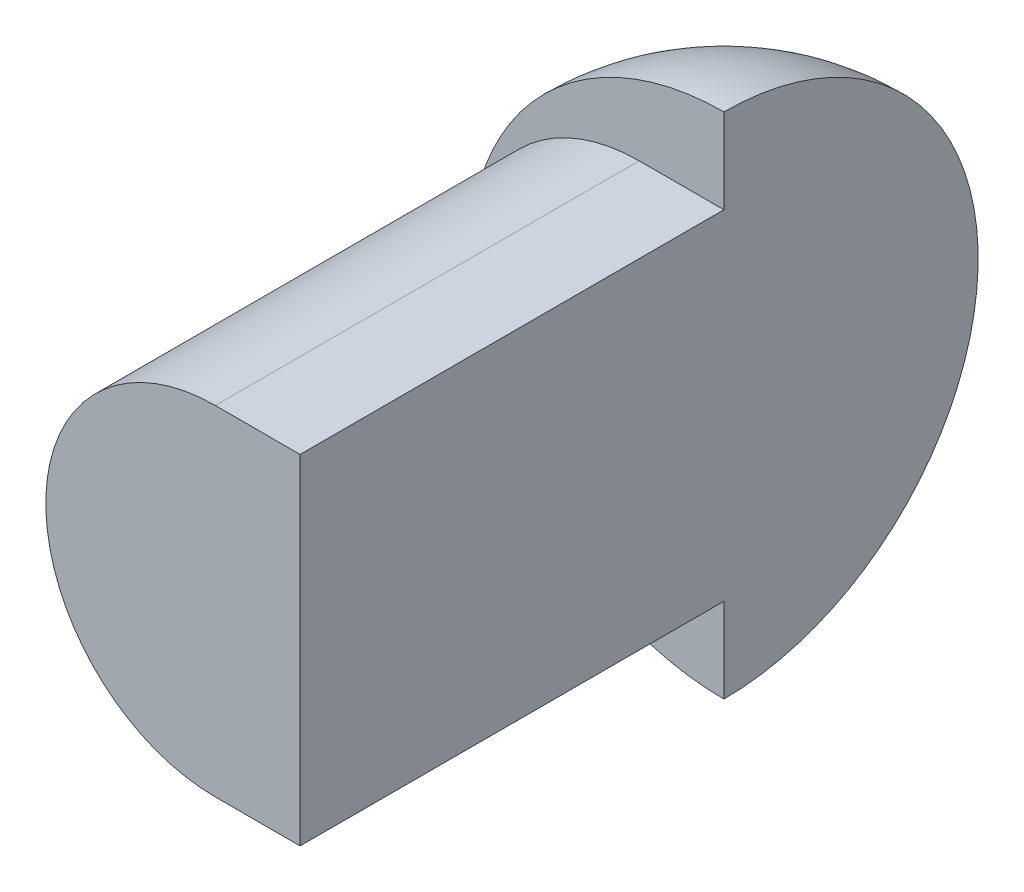
from build123d import *

# Parameters (mm, degrees)
EXTRUDE_1_DEPTH = 100
REVOLVE_1_ANGLE = 90


with BuildPart() as part:
    # 草图1 → 凸台-拉伸1 (new body)
    with BuildSketch(Plane.XY):
        with BuildLine():
            Line((0, 0), (0, -80))
            Line((0, -80), (-20, -80))
            ThreePointArc((-20, -80), (-60, -40), (-20, 0))
            Line((-20, 0), (0, 0))
        make_face()
    extrude(amount=-EXTRUDE_1_DEPTH)

    # 草图2 → 旋转1 (revolve)
    with BuildSketch(Plane(origin=(0, 0, 0), x_dir=(0, 0, -1), z_dir=(1, 0, 0))):
        with BuildLine():
            Line((100, 20), (100, -100))
            ThreePointArc((100, -100), (160, -40), (100, 20))
        make_face()
    revolve(axis=Axis((0, 20, -100), (0, 1, 0)), revolution_arc=REVOLVE_1_ANGLE)


solid = part.part
